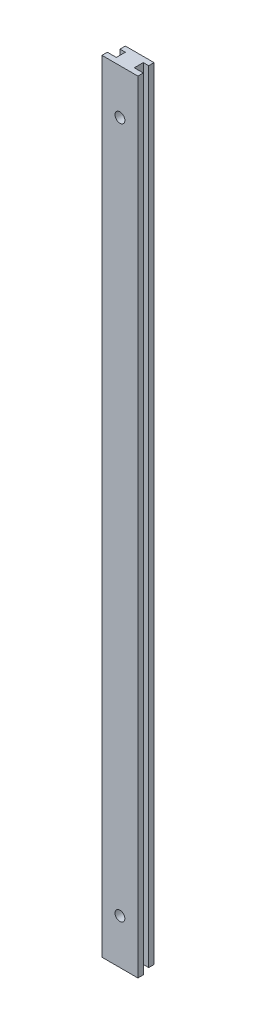
from build123d import *

# Parameters (mm, degrees)
BOSS_EXTRUDE1_DEPTH = 435
SKETCH2_R           = 2.75
CUT_EXTRUDE1_DEPTH  = 5


with BuildPart() as part:
    # Sketch1 → Boss-Extrude1 (new body)
    with BuildSketch(Plane(origin=(0, 0, 0), x_dir=(1, 0, 0), z_dir=(0, 1, 0))):
        Polygon((0, 0), (20, 0), (20, 3), (15, 3), (15, 8), (18, 8), (18, 11), (2, 11), (2, 8), (5, 8), (5, 3), (0, 3), align=None)
    extrude(amount=BOSS_EXTRUDE1_DEPTH)

    # Sketch2 → Cut-Extrude1 (cut)
    with BuildSketch(Plane.XY):
        with Locations((10, 410)):
            Circle(SKETCH2_R)
        with Locations((10, 25)):
            Circle(SKETCH2_R)
    extrude(amount=-CUT_EXTRUDE1_DEPTH, mode=Mode.SUBTRACT)


solid = part.part
